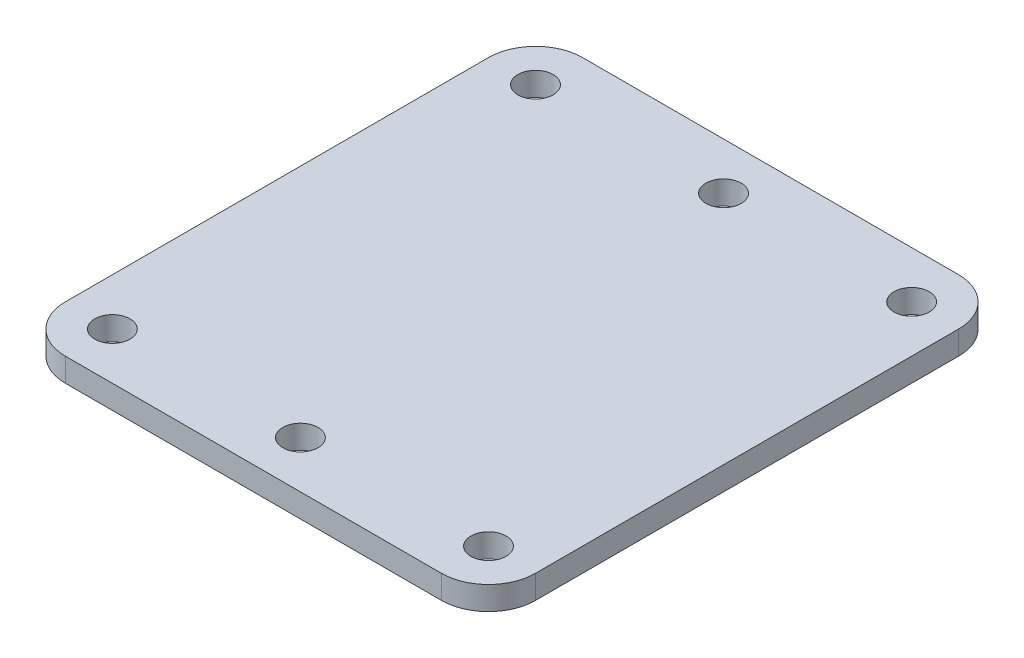
SolidWorks part; units mm, degrees
ref_plane "Front Plane" through (0, 0, 0) normal (0, 0, 1) x (1, 0, 0)
ref_plane "Top Plane" through (0, 0, 0) normal (0, 1, 0) x (1, 0, 0)
ref_plane "Right Plane" through (0, 0, 0) normal (1, 0, 0) x (0, 0, -1)
sketch "Sketch1" plane through (0, 0, 0) normal (0, 1, 0) x (1, 0, 0)
  line L1 (-100, 110) -> (100, 110)
  line L2 (-100, 110) -> (-100, -110)
  line L3 (-100, -110) -> (100, -110)
  line L4 (100, 110) -> (100, -110)
  line L5 (-100, 110) -> (100, -110) construction
  line L6 (-100, -110) -> (100, 110) construction
  point P0 (0, 0)
  dimension "D1" = 220
  dimension "D2" = 200
extrude "Boss-Extrude1" add sketch "Sketch1" along normal mid plane 10
sketch "Sketch2" plane through (0, 5, 0) normal (0, 1, 0) x (1, 0, 0)
  line L0 (0, 90) -> (0, -90) construction
  line L1 (80, 90) -> (-80, 90) construction
  line L2 (80, 90) -> (80, -90) construction
  line L3 (80, -90) -> (-80, -90) construction
  line L4 (-80, 90) -> (-80, -90) construction
  line L5 (80, 90) -> (-80, -90) construction
  line L6 (80, -90) -> (-80, 90) construction
  circle A0 centre (80, 90) radius 7.5
  point P0 (0, 0)
  dimension "D3" = 15
  dimension "D1" = 180
  dimension "D2" = 160
extrude "Cut-Extrude1" cut sketch "Sketch2" against normal blind 10
pattern_linear "LPattern1" count 2 spacing 180 along (0, 0, 1) count 3 spacing 80 along (-1, 0, 0) of "Cut-Extrude1"
fillet "Fillet1" radius 20 4 edges at (-100, 0, -110) (-100, 0, 110) (100, 0, 110) (100, 0, -110)
